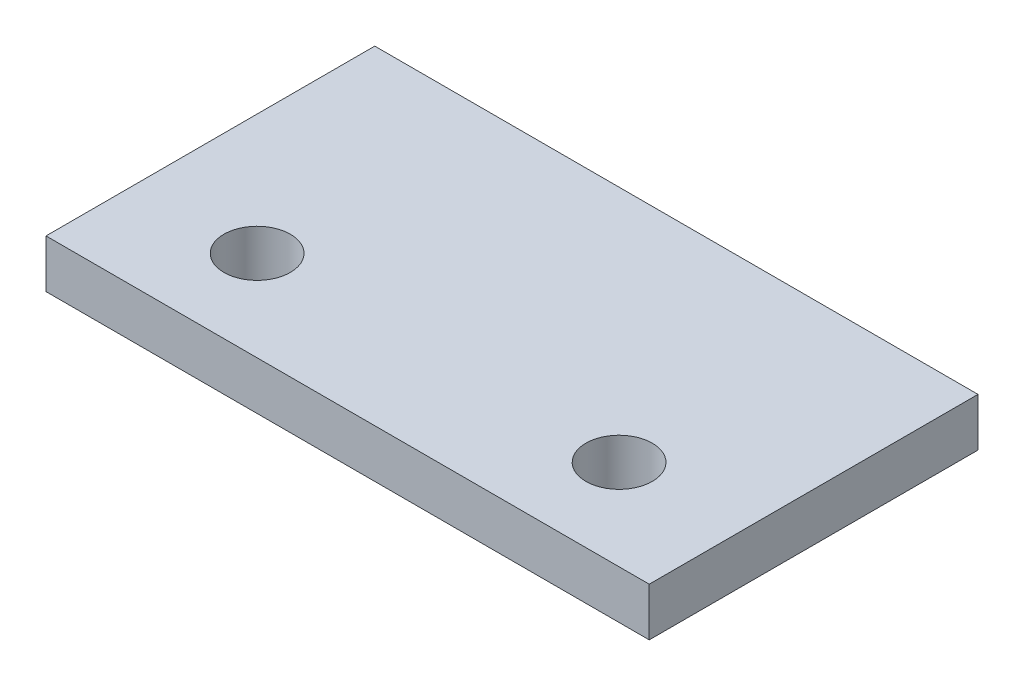
from build123d import *

# Parameters (mm, degrees)
SKETCH1_W                  = 100
SKETCH1_H                  = 54.5
BOSS_EXTRUDE1_DEPTH        = 8
F_11_0_11_DIAMETER_HOLE1_D = 11


with BuildPart() as part:
    # Sketch1 → Boss-Extrude1 (new body)
    with BuildSketch(Plane(origin=(0, 0, 0), x_dir=(1, 0, 0), z_dir=(0, 1, 0))):
        Rectangle(SKETCH1_W, SKETCH1_H)
    extrude(amount=BOSS_EXTRUDE1_DEPTH)

    # Ø11.0 (11) Diameter Hole1 (through all)
    with Locations(Plane(origin=(0, 8, 0), x_dir=(1, 0, 0), z_dir=(0, 1, 0))):
        with Locations((-30, -12.25), (30, -12.25)):
            Hole(F_11_0_11_DIAMETER_HOLE1_D / 2)


solid = part.part
